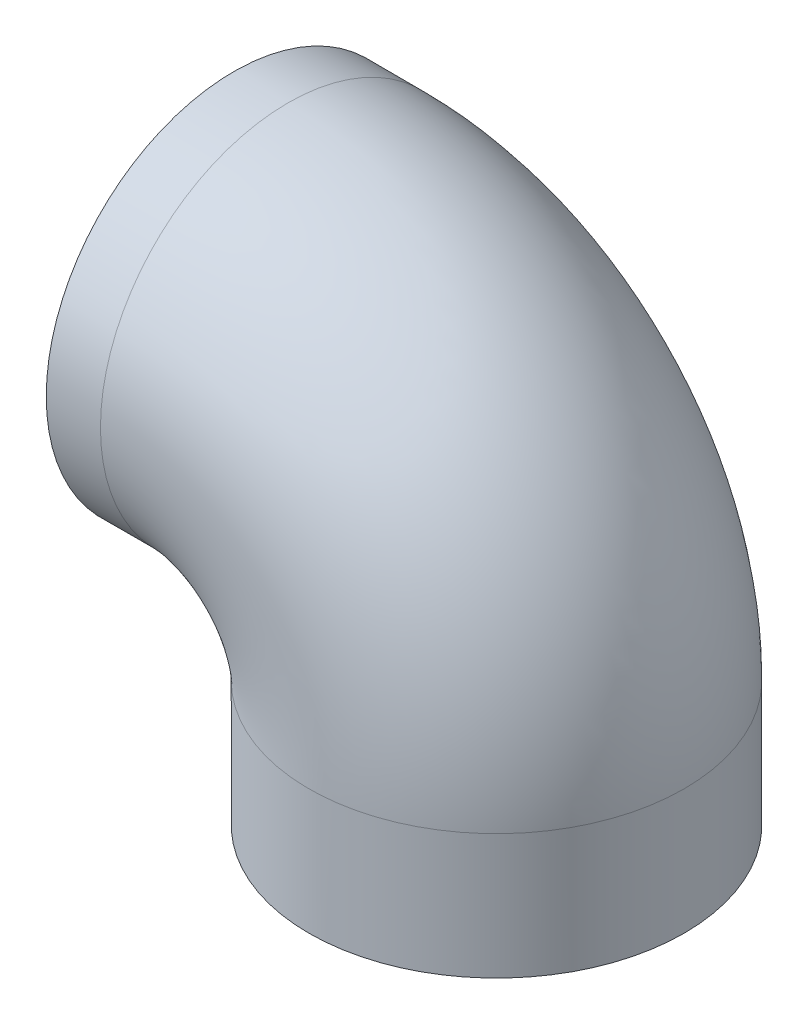
from build123d import *

# Parameters (mm, degrees)
SKETCH1_R           = 450
SKETCH1_R_2         = 400
BOSS_EXTRUDE1_DEPTH = 750
SKETCH2_R           = 650
BOSS_EXTRUDE2_DEPTH = 100
SKETCH3_R           = 50
CUT_EXTRUDE1_DEPTH  = 1846.264208725
MOVE_FACE1_BY       = 750
SKETCH9_R           = 450
SKETCH9_R_2         = 400
SKETCH11_R          = 1265.740496662
CUT_EXTRUDE2_DEPTH  = 3153
MOVE_FACE2_BY       = 370
MOVE_FACE3_BY       = 200


with BuildPart() as part:
    # Sketch1 → Boss-Extrude1 (new, symmetric)
    with BuildSketch(Plane(origin=(0, 0, 0), x_dir=(1, 0, 0), z_dir=(0, 1, 0))):
        with Locations(Location((0, 0, 0), (0, 0, 270))):
            Circle(SKETCH1_R)
        with Locations(Location((0, 0, 0), (0, 0, 270))):
            Circle(SKETCH1_R_2, mode=Mode.SUBTRACT)
    extrude(amount=BOSS_EXTRUDE1_DEPTH, both=True)

    # Sketch2 → Boss-Extrude2 (add)
    with BuildSketch(Plane.XZ.offset(750)):
        with Locations(Location((0, 0, 0), (0, 0, 270))):
            Circle(SKETCH2_R)
    extrude(amount=BOSS_EXTRUDE2_DEPTH)

    # Sketch3 → Cut-Extrude1 (cut, through all)
    with BuildSketch(Plane.XZ.offset(850)):
        with Locations(Location((0, 550, 0), (0, 0, 270))):
            Circle(SKETCH3_R)
        with Locations(Location((550, 0, 0), (0, 0, 270))):
            Circle(SKETCH3_R)
        with Locations(Location((0, -550, 0), (0, 0, 270))):
            Circle(SKETCH3_R)
        with Locations(Location((-550, 0, 0), (0, 0, 270))):
            Circle(SKETCH3_R)
    extrude(amount=-CUT_EXTRUDE1_DEPTH, mode=Mode.SUBTRACT)

    # Move Face1: a face moved inward by 750.0
    extrude(part.faces().sort_by_distance((-225, 750, 360))[0], amount=MOVE_FACE1_BY, dir=(0, -1, 0), mode=Mode.SUBTRACT)

    # Sweep1: sweep along a path in Sketch8
    with BuildLine(Plane.XY) as sweep1_path:
        Line((0, 0), (0, 500))
        ThreePointArc((0, 500), (-146.446609407, 853.553390593), (-500, 1000))
        Line((-500, 1000), (-1000, 1000))
    # Sketch9 → Sweep1 (sweep)
    with BuildSketch(Plane(origin=(0, 0, 0), x_dir=(1, 0, 0), z_dir=(0, 1, 0))):
        Circle(SKETCH9_R)
        Circle(SKETCH9_R_2, mode=Mode.SUBTRACT)
    sweep(path=sweep1_path.line)

    # Sketch11 → Cut-Extrude2 (cut)
    with BuildSketch(Plane(origin=(0, 0, 0), x_dir=(1, 0, 0), z_dir=(0, 1, 0))):
        with Locations((-18.825691705, 0)):
            Circle(SKETCH11_R)
    extrude(amount=-CUT_EXTRUDE2_DEPTH, mode=Mode.SUBTRACT)

    # Move Face2: a face moved inward by 370.0
    extrude(part.faces().sort_by_distance((-1000, 1360, 225))[0], amount=MOVE_FACE2_BY, dir=(1, 0, 0), mode=Mode.SUBTRACT)

    # Move Face3: a face moved inward by 200.0
    extrude(part.faces().sort_by_distance((-225, 0, 360))[0], amount=MOVE_FACE3_BY, dir=(0, 1, 0), mode=Mode.SUBTRACT)


solid = part.part
